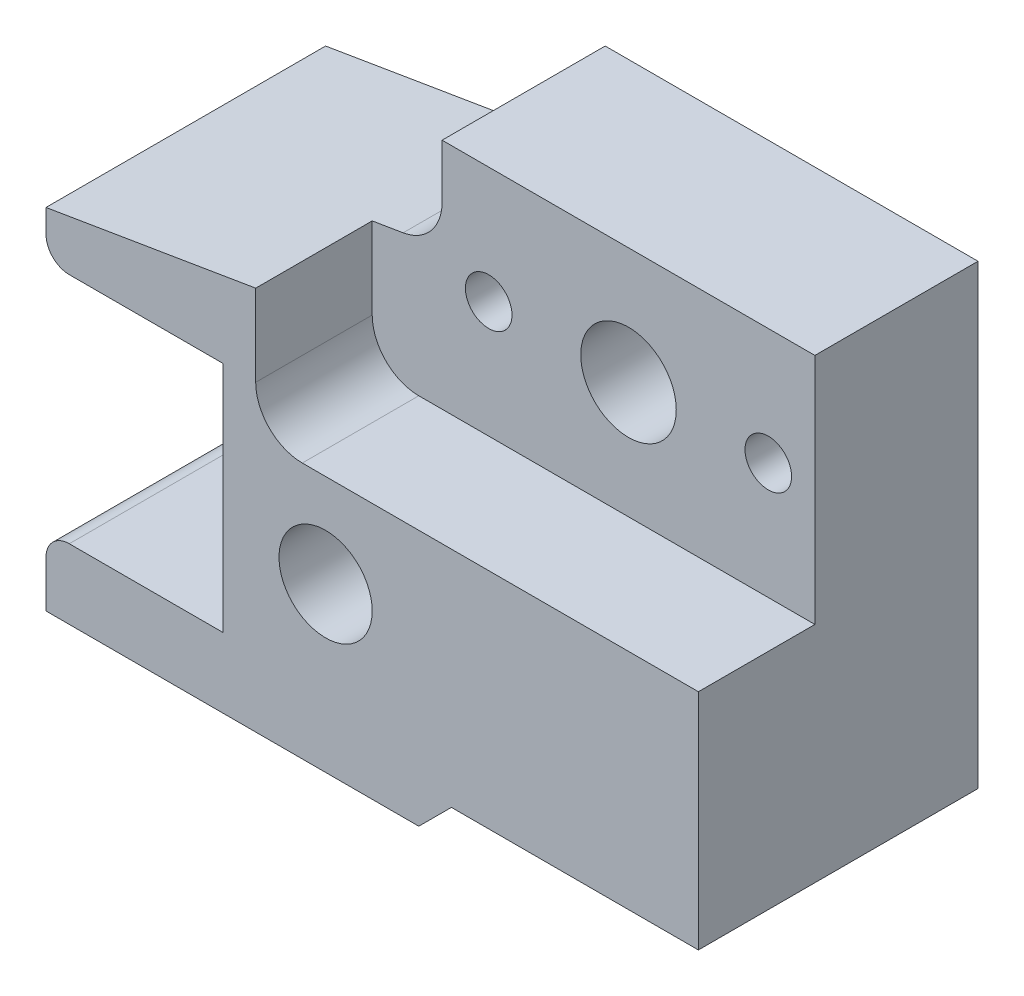
from build123d import *

# Parameters (mm, degrees)
SKETCH1_W                    = 14
SKETCH1_H                    = 10.5
BOSS_EXTRUDE1_DEPTH          = 3
SKETCH2_W                    = 9.5
SKETCH2_H                    = 5
CUT_EXTRUDE1_DEPTH           = 2.5
CUT_EXTRUDE2_DEPTH           = 11.609547587
FILLET1_R                    = 1
SKETCH4_W                    = 3.8
SKETCH4_H                    = 5
CUT_EXTRUDE3_DEPTH           = 11.609547587
M2_5_TAPPED_HOLE1_D          = 2.05
F_1_0_1_DIAMETER_HOLE1_D     = 1
F_2_0_2_DIAMETER_HOLE1_D     = 2
CUT_EXTRUDE4_DEPTH           = 11.609547587
F_3_0_3_DIAMETER_HOLE1_D     = 3
F_3_0_3_DIAMETER_HOLE1_DEPTH = 4
F_3_0_3_DIAMETER_HOLE1_TIP   = 0.901290929
FILLET2_R                    = 0.5
M2_5_TAPPED_HOLE2_D          = 2.05
M2_5_TAPPED_HOLE2_DEPTH      = 4
M2_5_TAPPED_HOLE2_TIP        = 0.615882135


with BuildPart() as part:
    # Sketch1 → Boss-Extrude1 (new, symmetric)
    with BuildSketch(Plane.XY):
        Rectangle(SKETCH1_W, SKETCH1_H)
    extrude(amount=BOSS_EXTRUDE1_DEPTH, both=True)

    # Sketch2 → Cut-Extrude1 (cut)
    with BuildSketch(Plane.XY.offset(3)):
        with Locations((2.25, 2.75)):
            Rectangle(SKETCH2_W, SKETCH2_H)
    extrude(amount=-CUT_EXTRUDE1_DEPTH, mode=Mode.SUBTRACT)

    # Sketch3 → Cut-Extrude2 (cut, through all)
    with BuildSketch(Plane.XY.offset(3)):
        Polygon((-7, 5.25), (-1, 5.25), (-1, 3.25), (-7, 2.25), align=None)
    extrude(amount=-CUT_EXTRUDE2_DEPTH, mode=Mode.SUBTRACT)

    # Fillet1
    fillet1_edges = [part.edges().sort_by_distance(p)[0] for p in [
        (-2.5, 0.25, 1.75),
        (-1, 3.25, -1.25),
    ]]
    fillet(fillet1_edges, radius=FILLET1_R)

    # Sketch4 → Cut-Extrude3 (cut, through all)
    with BuildSketch(Plane.XY.offset(3)):
        with Locations((-5.1, -1.25)):
            Rectangle(SKETCH4_W, SKETCH4_H)
    extrude(amount=-CUT_EXTRUDE3_DEPTH, mode=Mode.SUBTRACT)

    # M2.5 Tapped Hole1 (through all)
    with Locations(Plane.XY.offset(0.5)):
        with Locations((3, 2.75)):
            Hole(M2_5_TAPPED_HOLE1_D / 2)

    # Ø1.0 (1) Diameter Hole1 (through all)
    with Locations(Plane.XY.offset(0.5)):
        with Locations((0, 2.75), (6, 2.75)):
            Hole(F_1_0_1_DIAMETER_HOLE1_D / 2)

    # Ø2.0 (2) Diameter Hole1 (through all)
    with Locations(Plane.XY.offset(3)):
        with Locations((-1, -1.75)):
            Hole(F_2_0_2_DIAMETER_HOLE1_D / 2)

    # Sketch15 → Cut-Extrude4 (cut, through all)
    with BuildSketch(Plane.XY.offset(3)):
        Polygon((7, -5.25), (1, -5.25), (1.7, -4.55), (7, -4.55), align=None)
    extrude(amount=-CUT_EXTRUDE4_DEPTH, mode=Mode.SUBTRACT)

    # Ø3.0 (3) Diameter Hole1
    with Locations(Plane(origin=(0, -4.55, 0), x_dir=(-1, 0, 0), z_dir=(0, -1, 0))):
        with Locations((-4.2, 0)):
            Hole(F_3_0_3_DIAMETER_HOLE1_D / 2, depth=F_3_0_3_DIAMETER_HOLE1_DEPTH)
            with Locations((0, 0, -(F_3_0_3_DIAMETER_HOLE1_DEPTH + F_3_0_3_DIAMETER_HOLE1_TIP / 2))):  # 118° drill point
                Cone(0, F_3_0_3_DIAMETER_HOLE1_D / 2, F_3_0_3_DIAMETER_HOLE1_TIP, mode=Mode.SUBTRACT)

    # Fillet2
    fillet2_edges = [part.edges().sort_by_distance(p)[0] for p in [
        (-7, -3.75, 0),
        (-7, 1.25, 0),
    ]]
    fillet(fillet2_edges, radius=FILLET2_R)

    # M2.5 Tapped Hole2
    with Locations(Plane(origin=(0, -5.25, 0), x_dir=(-1, 0, 0), z_dir=(0, -1, 0))):
        with Locations((1, 0)):
            Hole(M2_5_TAPPED_HOLE2_D / 2, depth=M2_5_TAPPED_HOLE2_DEPTH)
            with Locations((0, 0, -(M2_5_TAPPED_HOLE2_DEPTH + M2_5_TAPPED_HOLE2_TIP / 2))):  # 118° drill point
                Cone(0, M2_5_TAPPED_HOLE2_D / 2, M2_5_TAPPED_HOLE2_TIP, mode=Mode.SUBTRACT)


solid = part.part
